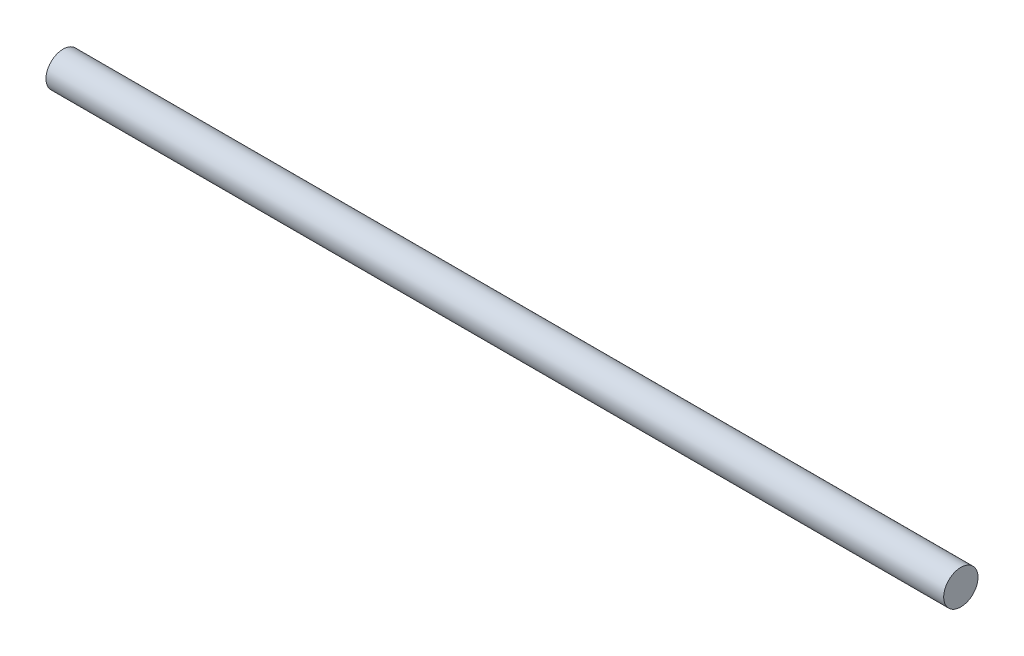
from build123d import *

# Parameters (mm, degrees)
SKETCH1_R           = 6.5
BOSS_EXTRUDE1_DEPTH = 170


with BuildPart() as part:
    # Sketch1 → Boss-Extrude1 (new, symmetric)
    with BuildSketch(Plane(origin=(0, 0, 0), x_dir=(0, 0, -1), z_dir=(1, 0, 0))):
        Circle(SKETCH1_R)
    extrude(amount=BOSS_EXTRUDE1_DEPTH, both=True)


solid = part.part
